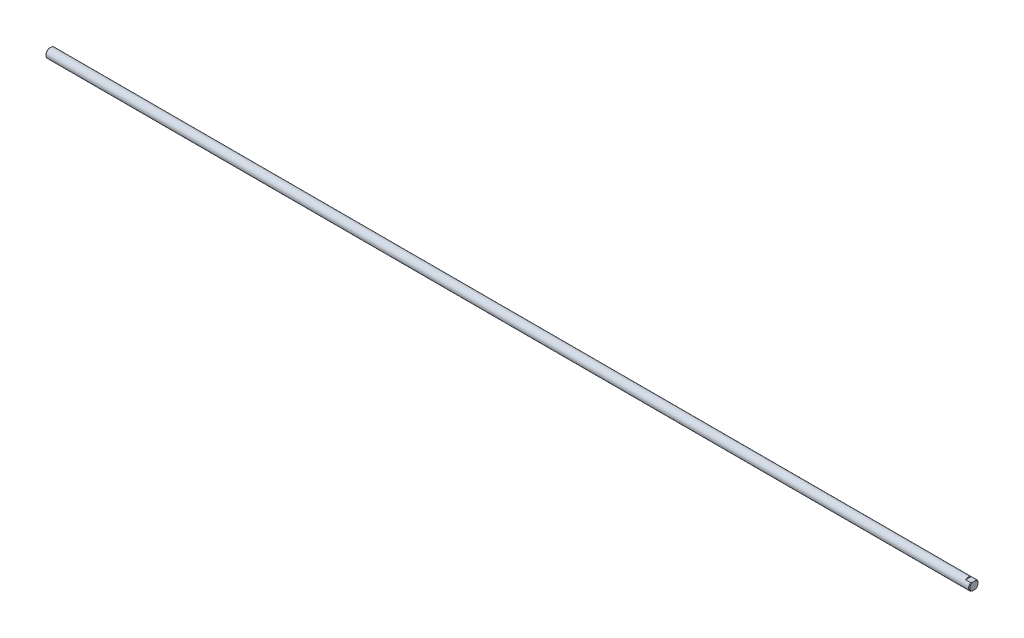
SolidWorks part; units mm, degrees
material "普通碳钢"
ref_plane "Front Plane" through (0, 0, 0) normal (0, 0, 1) x (1, 0, 0)
ref_plane "Top Plane" through (0, 0, 0) normal (0, 1, 0) x (1, 0, 0)
ref_plane "Right Plane" through (0, 0, 0) normal (1, 0, 0) x (0, 0, -1)
sketch "Sketch1" plane through (0, 0, 0) normal (1, 0, 0) x (0, 0, -1)
  circle A0 centre (0, 0) radius 7.5
  dimension "D1" = 15
extrude "Boss-Extrude1" add sketch "Sketch1" along normal blind 1480
hole_wizard "M5 Tapped Hole1" positions "Sketch4" profile "Sketch5" tap size "M5" standard "GB"
sketch "Sketch4" plane through (0, 0, 0) normal (-1, 0, 0) x (0, 0, 1)
  point P0 (0, 0)
sketch "Sketch5" plane through (0, 0, 0) normal (0, 1, 0) x (0, 0, 1)
  line L0 (0, 0) -> (0, 13.6618)
  line L1 (0, 13.6618) -> (2.1, 12.4)
  line L2 (2.1, 12.4) -> (2.1, 0)
  line L5 (2.1, 0) -> (0, 0)
  line L10 (0, 13.6618) -> (-2.1, 12.4) construction
  line L11 (0, -6.35) -> (0, 107.95) construction
  dimension "螺纹孔钻头直径" = 4.2
  dimension "螺纹孔钻头深度" = 12.4
  dimension "导头角度" = 118
cosmetic thread "Hole thread 1" [suppressed] parameters "D1"=10, "D2"=5
hole_wizard "M5 Tapped Hole2" positions "Sketch6" profile "Sketch7" tap size "M5" standard "GB"
sketch "Sketch6" plane through (275, 0, 0) normal (1, 0, 0) x (0, 0, -1)
  point P0 (0, 0)
sketch "Sketch7" plane through (275, 0, 0) normal (0, 1, 0) x (0, 0, -1)
  line L0 (0, 0) -> (0, 13.6618)
  line L1 (0, 13.6618) -> (2.1, 12.4)
  line L2 (2.1, 12.4) -> (2.1, 0)
  line L5 (2.1, 0) -> (0, 0)
  line L10 (0, 13.6618) -> (-2.1, 12.4) construction
  line L11 (0, -6.35) -> (0, 107.95) construction
  dimension "螺纹孔钻头直径" = 4.2
  dimension "螺纹孔钻头深度" = 12.4
  dimension "导头角度" = 118
cosmetic thread "Hole thread 2" [suppressed] parameters "D1"=10, "D2"=5
chamfer "Chamfer1" distance 1 angle 45 2 edges at (0, 0, -7.5) (1480, 0, -7.5)
sketch "Sketch8" plane through (0, 0, 0) normal (0, 0, 1) x (1, 0, 0)
  line L0 (1480, 0) -> (271.6406, 0) construction
  line L1 (1514.5673, 7.8996) -> (1471, 7.8996)
  line L2 (1514.5673, 7.8996) -> (1514.5673, 6)
  line L3 (1514.5673, 6) -> (1471, 6)
  line L4 (1471, 7.8996) -> (1471, 6)
  line L5 (1480, -7.5) -> (1480, 7.5) construction
  line L6 (1471, -7.8996) -> (1471, -6)
  line L7 (1514.5673, -6) -> (1471, -6)
  line L8 (1514.5673, -7.8996) -> (1514.5673, -6)
  line L9 (1514.5673, -7.8996) -> (1471, -7.8996)
  dimension "D1" = 12
  dimension "D2" = 9
extrude "Cut-Extrude1" cut sketch "Sketch8" against normal through all both and the other way through all
